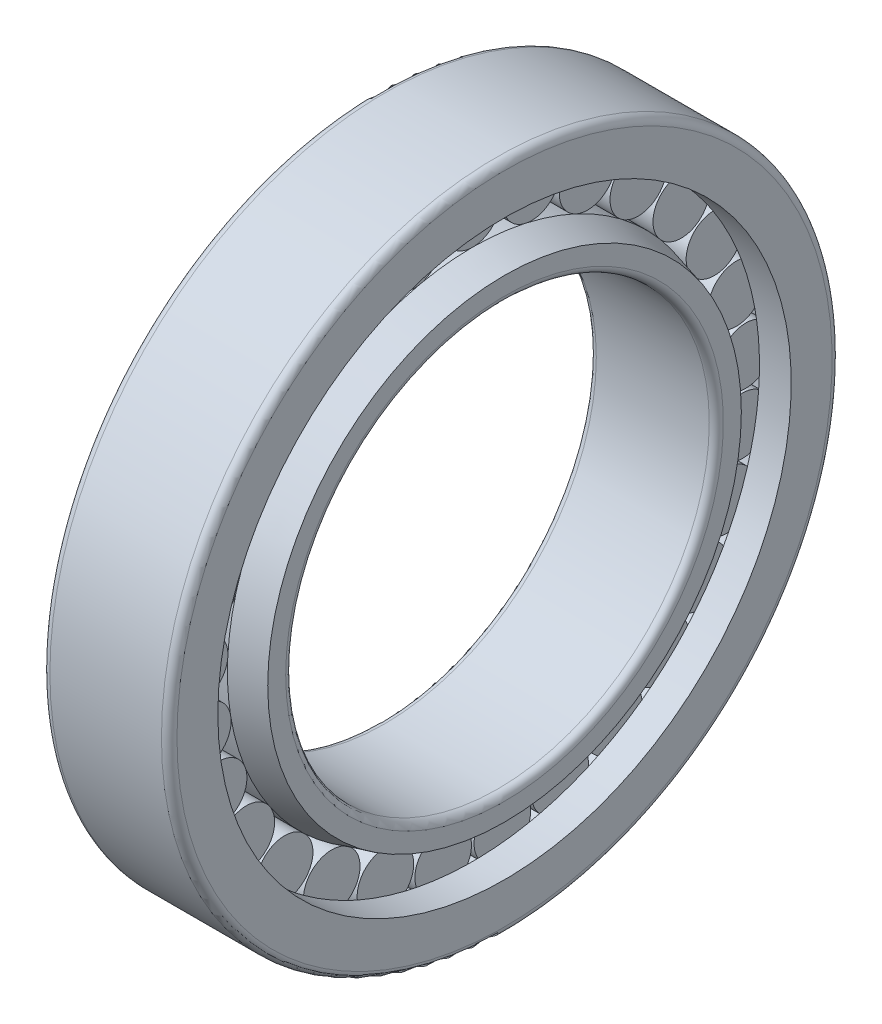
SolidWorks part; units mm, degrees
ref_plane "Front" through (0, 0, 0) normal (0, 0, 1) x (1, 0, 0)
ref_plane "Top" through (0, 0, 0) normal (0, 1, 0) x (1, 0, 0)
ref_plane "Right" through (0, 0, 0) normal (1, 0, 0) x (0, 0, -1)
other "Configuration Table"
sketch "Sketch1" plane through (0, 0, 0) normal (0, 0, 1) x (1, 0, 0)
  line L0 (-9, 30) -> (9, 30)
  line L1 (9, 30) -> (9, 33.5442)
  line L2 (9, 33.5442) -> (4.5, 34.75)
  line L3 (4.5, 34.75) -> (-4.5, 34.75)
  line L4 (-4.5, 34.75) -> (-9, 33.5442)
  line L5 (-9, 33.5442) -> (-9, 30)
  line L6 (-10.1379, 0) -> (10.5422, 0) construction
revolve "Revolve1" add sketch "Sketch1" angle 360 about L6
sketch "Sketch2" plane through (0, 0, 0) normal (0, 0, 1) x (1, 0, 0)
  line L0 (-4.5, 34.74) -> (4.5, 34.74)
  line L1 (4.5, 34.74) -> (4.5, 38.75)
  line L2 (-4.5, 38.75) -> (4.5, 38.75)
  line L3 (-4.5, 38.75) -> (-4.5, 34.74)
  line L4 (-7.1198, 0) -> (7.769, 0) construction
  line L6 (-7.4228, 38.75) -> (7.769, 38.75) construction
revolve "Revolve2" add sketch "Sketch2" angle 360 about L6
sketch "Sketch3" plane through (0, 0, 0) normal (0, 0, 1) x (1, 0, 0)
  line L0 (-9, 47.5) -> (9, 47.5)
  line L1 (9, 47.5) -> (9, 40.6125)
  line L2 (9, 40.6125) -> (4.49, 40.6125)
  line L3 (4.49, 40.6125) -> (4.49, 42.75)
  line L4 (4.49, 42.75) -> (-4.49, 42.75)
  line L5 (-4.49, 42.75) -> (-4.49, 40.6125)
  line L6 (-4.49, 40.6125) -> (-9, 40.6125)
  line L7 (-9, 40.6125) -> (-9, 47.5)
  line L8 (-9.0822, 0) -> (10.5352, 0) construction
revolve "Revolve3" add sketch "Sketch3" angle 360 about L8
pattern_circular "Circular-Pattern1" count 29 over 360 about axis through (0, 0, 0) along (1, 0, 0) of "Revolve2"
fillet "Fillet1" radius 1.1 2 edges at (-9, 0, 47.5) (9, 0, 47.5)
fillet "Fillet2" radius 1 2 edges at (9, 0, 30) (-9, 0, 30)
equation "\"D2@Sketch1\" = \"B@Sketch1\" / 2"
equation "\"D7@Sketch1\" = \"D2@Sketch1\""
equation "\"D8@Sketch1\" = \"D7@Sketch1\"/2"
equation "\"D2@Sketch2\" = ( \"DD@Sketch3\" + \"d@Sketch1\" )  / 4"
equation "\"D4@Sketch2\" = \"B@Sketch1\" / 2"
equation "\"D5@Sketch2\" = \"D4@Sketch2\" / 2"
equation "\"D1@Sketch2\" = \"FW@Sketch1\" - 0.02"
equation "\"B@Sketch3\" = \"B@Sketch1\""
equation "\"D5@Sketch3\" = \"B@Sketch3\" / 2"
equation "\"D6@Sketch3\" = \"D5@Sketch3\" - 0.02"
equation "\"D7@Sketch3\" = \"D6@Sketch3\" / 2"
equation "\"D2@Sketch3\" = ( \"DD@Sketch3\" + \"d@Sketch1\" )  / 4 * 2 + ( ( \"DD@Sketch3\" + \"d@Sketch1\" )  / 4 * 2 - \"FW@Sketch1\"  ) "
equation "\"D3@Sketch3\" = \"D2@Sketch3\" * 0.95"
equation "\"m@Circular-Pattern1\"=int(3.14159265/atn(((\"DD@Sketch3\"+\"d@Sketch1\")/4-\"FW@Sketch1\"/2+0.02) / sqr((\"DD@Sketch3\"+\"d@Sketch1\")/4  * (\"DD@Sketch3\"+\"d@Sketch1\")/4 - ((\"DD@Sketch3\"+\"d@Sketch1\")/4-\"FW@Sketch1\"/2+0.02) *  ((\"DD@Sketch3\"+\"d@Sketch1\")/4-\"FW@Sketch1\"/2+0.02))))-1"
